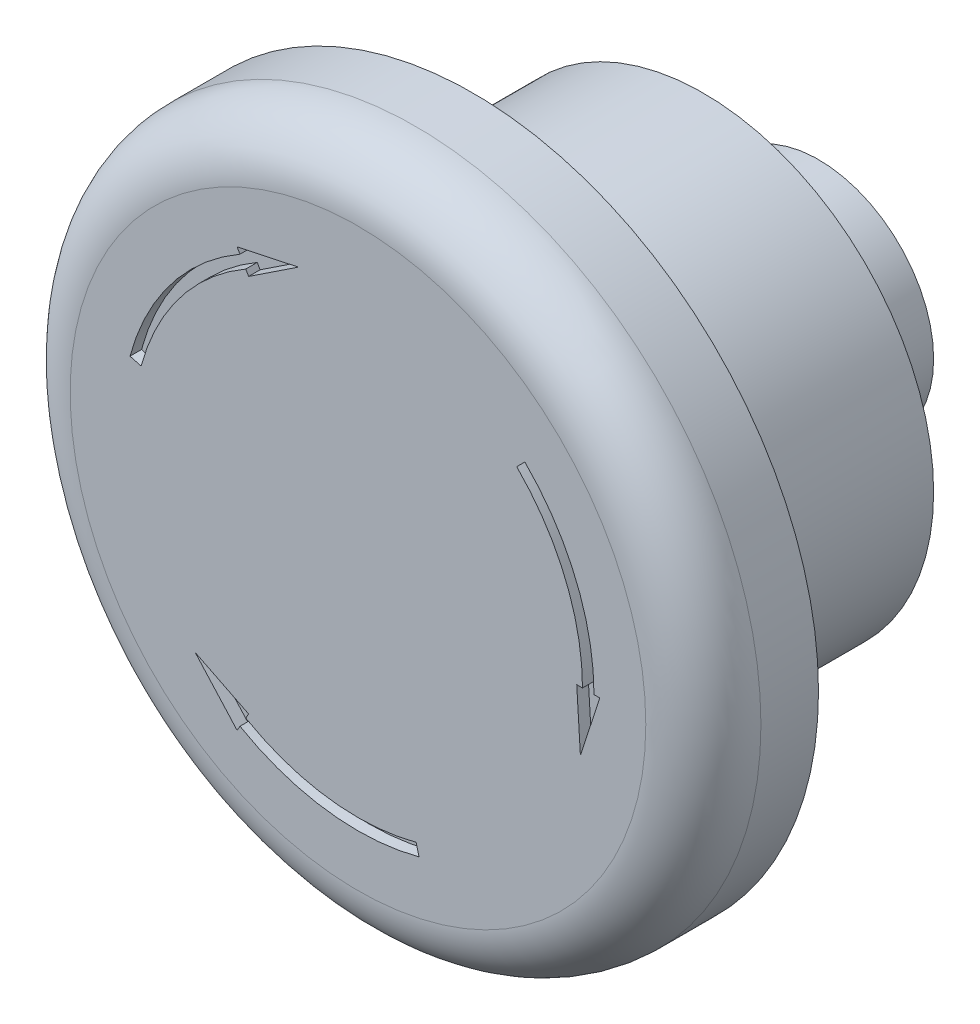
from build123d import *

# Parameters (mm, degrees)
SKETCH_1_R               = 100
EXTRUDE_1_DEPTH          = 100
SKETCH_2_R               = 200
EXTRUDE_2_DEPTH          = 200
SKETCH_3_R               = 300
EXTRUDE_3_DEPTH          = 100
CUT_EXTRUDE_1_DEPTH      = 10
PATTERN_CIRCULAR_1_COUNT = 3
FILLET_1_R               = 50
SCALE_1_SCALE            = 0.1


with BuildPart() as part:
    # 草图1 → 凸台-拉伸1 (new body)
    with BuildSketch(Plane.XY):
        Circle(SKETCH_1_R)
    extrude(amount=EXTRUDE_1_DEPTH)

    # 草图2 → 凸台-拉伸2 (add)
    with BuildSketch(Plane.XY.offset(100)):
        Circle(SKETCH_2_R)
    extrude(amount=EXTRUDE_2_DEPTH)

    # 草图3 → 凸台-拉伸3 (add)
    with BuildSketch(Plane.XY.offset(300)):
        Circle(SKETCH_3_R)
    extrude(amount=EXTRUDE_3_DEPTH)

    # 草图4 → 切除-拉伸1 (cut)
    with BuildSketch(Plane.XY.offset(400)):
        with BuildLine():
            Line((-188.355536126, 50.469713795), (-198.014794389, 53.057904246))
            ThreePointArc((-198.014794389, 53.057904246), (-162.63743476, 124.796092947), (-102.5, 177.535207776))
            Line((-102.5, 177.535207776), (-105, 181.865334795))
            Line((-105, 181.865334795), (-51.763809021, 193.185165258))
            Line((-51.763809021, 193.185165258), (-95, 164.544826719))
            Line((-95, 164.544826719), (-97.5, 168.874953738))
            ThreePointArc((-97.5, 168.874953738), (-154.703901357, 118.708478657), (-188.355536126, 50.469713795))
        make_face()
    cut_extrude_1 = extrude(amount=-CUT_EXTRUDE_1_DEPTH, mode=Mode.SUBTRACT)

    # 阵列(圆周)1: 切除-拉伸1 ×3 about axis
    pattern_circular_1_axis = Axis((0, 0, 0), (0, 0, 1))
    for i in range(1, PATTERN_CIRCULAR_1_COUNT):
        add(cut_extrude_1.rotate(pattern_circular_1_axis, i * 360 / PATTERN_CIRCULAR_1_COUNT), mode=Mode.SUBTRACT)

    # 圆角1
    fillet_1_edges = [part.edges().sort_by_distance(p)[0] for p in [
        (-300, 0, 400),
    ]]
    fillet(fillet_1_edges, radius=FILLET_1_R)


with BuildPart() as part_1:
    # 缩放比例1: scaled about (0, 0, 264.382298041)
    add(part.part.scale(SCALE_1_SCALE).moved(Location((0, 0, 237.944068237))))


solid = part_1.part
